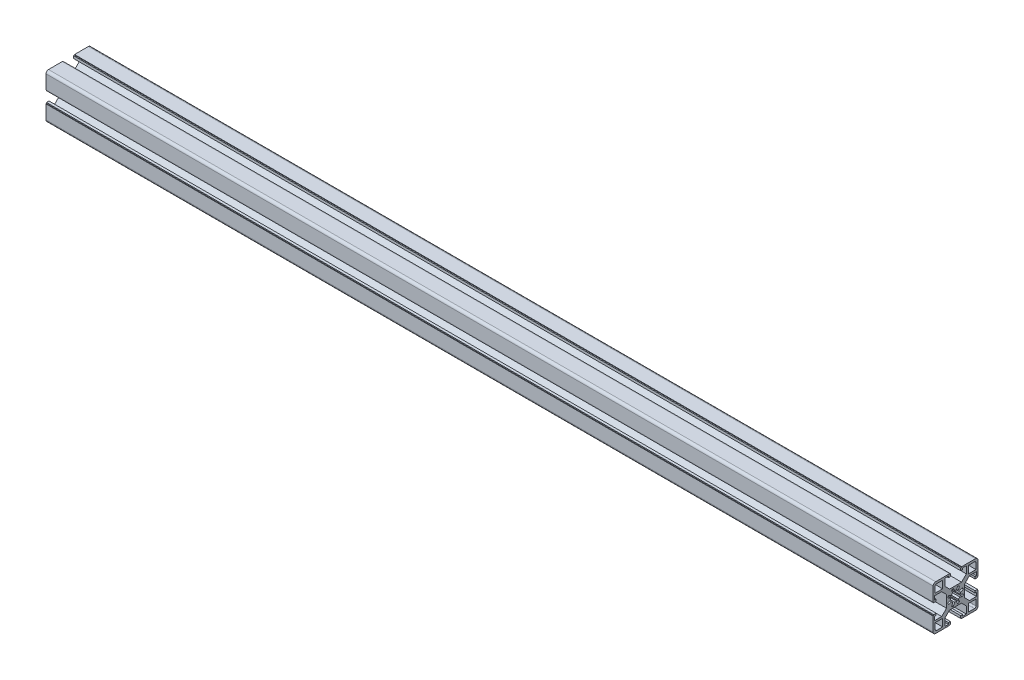
from build123d import *

# Parameters (mm, degrees)
ALUMINUM_PROFILE_45_X_45L_X_R2_5_1_DEPTH = 890


with BuildPart() as part:
    # Sketch1 → Aluminum Profile 45 X 45L X R2.5(1) (new body)
    with BuildSketch(Plane.YZ):
        with BuildLine():
            Line((6.1, -22.5), (20, -22.5))
            ThreePointArc((20, -22.5), (21.767766953, -21.767766953), (22.5, -20))
            Line((22.5, -20), (22.5, -6.1))
            Line((22.5, -6.1), (22, -6.1))
            Line((22, -6.1), (22, -5.1))
            Line((22, -5.1), (19.5, -5.1))
            Line((19.5, -5.1), (19.5, -7.1))
            Line((19.5, -7.1), (21, -7.1))
            Line((21, -7.1), (21, -10.8))
            Line((21, -10.8), (13.9, -10.8))
            Line((13.9, -10.8), (9.1, -6))
            Line((9.1, -6), (9.1, 6))
            Line((9.1, 6), (13.9, 10.8))
            Line((13.9, 10.8), (21, 10.8))
            Line((21, 10.8), (21, 7.1))
            Line((21, 7.1), (19.5, 7.1))
            Line((19.5, 7.1), (19.5, 5.1))
            Line((19.5, 5.1), (22, 5.1))
            Line((22, 5.1), (22, 6.1))
            Line((22, 6.1), (22.5, 6.1))
            Line((22.5, 6.1), (22.5, 20))
            ThreePointArc((22.5, 20), (21.767766953, 21.767766953), (20, 22.5))
            Line((20, 22.5), (6.1, 22.5))
            Line((6.1, 22.5), (6.1, 22))
            Line((6.1, 22), (5.1, 22))
            Line((5.1, 22), (5.1, 19.5))
            Line((5.1, 19.5), (7.1, 19.5))
            Line((7.1, 19.5), (7.1, 21))
            Line((7.1, 21), (10.8, 21))
            Line((10.8, 21), (10.8, 13.9))
            Line((10.8, 13.9), (6, 9.1))
            Line((6, 9.1), (-6, 9.1))
            Line((-6, 9.1), (-10.8, 13.9))
            Line((-10.8, 13.9), (-10.8, 21))
            Line((-10.8, 21), (-7.1, 21))
            Line((-7.1, 21), (-7.1, 19.5))
            Line((-7.1, 19.5), (-5.1, 19.5))
            Line((-5.1, 19.5), (-5.1, 22))
            Line((-5.1, 22), (-6.1, 22))
            Line((-6.1, 22), (-6.1, 22.5))
            Line((-6.1, 22.5), (-20, 22.5))
            ThreePointArc((-20, 22.5), (-21.767766953, 21.767766953), (-22.5, 20))
            Line((-22.5, 20), (-22.5, 6.1))
            Line((-22.5, 6.1), (-22, 6.1))
            Line((-22, 6.1), (-22, 5.1))
            Line((-22, 5.1), (-19.5, 5.1))
            Line((-19.5, 5.1), (-19.5, 7.1))
            Line((-19.5, 7.1), (-21, 7.1))
            Line((-21, 7.1), (-21, 10.8))
            Line((-21, 10.8), (-13.9, 10.8))
            Line((-13.9, 10.8), (-9.1, 6))
            Line((-9.1, 6), (-9.1, -6))
            Line((-9.1, -6), (-13.9, -10.8))
            Line((-13.9, -10.8), (-21, -10.8))
            Line((-21, -10.8), (-21, -7.1))
            Line((-21, -7.1), (-19.5, -7.1))
            Line((-19.5, -7.1), (-19.5, -5.1))
            Line((-19.5, -5.1), (-22, -5.1))
            Line((-22, -5.1), (-22, -6.1))
            Line((-22, -6.1), (-22.5, -6.1))
            Line((-22.5, -6.1), (-22.5, -20))
            ThreePointArc((-22.5, -20), (-21.767766953, -21.767766953), (-20, -22.5))
            Line((-20, -22.5), (-6.1, -22.5))
            Line((-6.1, -22.5), (-6.1, -22))
            Line((-6.1, -22), (-5.1, -22))
            Line((-5.1, -22), (-5.1, -19.5))
            Line((-5.1, -19.5), (-7.1, -19.5))
            Line((-7.1, -19.5), (-7.1, -21))
            Line((-7.1, -21), (-10.8, -21))
            Line((-10.8, -21), (-10.8, -13.9))
            Line((-10.8, -13.9), (-6, -9.1))
            Line((-6, -9.1), (6, -9.1))
            Line((6, -9.1), (10.8, -13.9))
            Line((10.8, -13.9), (10.8, -21))
            Line((10.8, -21), (7.1, -21))
            Line((7.1, -21), (7.1, -19.5))
            Line((7.1, -19.5), (5.1, -19.5))
            Line((5.1, -19.5), (5.1, -22))
            Line((5.1, -22), (6.1, -22))
            Line((6.1, -22), (6.1, -22.5))
        make_face()
        with BuildLine():
            Line((-12.8, 20.5), (-18.8, 20.5))
            ThreePointArc((-18.8, 20.5), (-19.860660172, 20.060660172), (-20.3, 19))
            Line((-20.3, 19), (-20.3, 13))
            Line((-20.3, 13), (-12.8, 13))
            Line((-12.8, 13), (-12.8, 20.5))
        make_face(mode=Mode.SUBTRACT)
        with BuildLine():
            Line((-20.3, -13), (-20.3, -19))
            ThreePointArc((-20.3, -19), (-19.860660172, -20.060660172), (-18.8, -20.5))
            Line((-18.8, -20.5), (-12.8, -20.5))
            Line((-12.8, -20.5), (-12.8, -13))
            Line((-12.8, -13), (-20.3, -13))
        make_face(mode=Mode.SUBTRACT)
        with BuildLine():
            Line((7.008352828, 3.985346991), (4.143383445, 2.798637817))
            ThreePointArc((4.143383445, 2.798637817), (3.535533906, 3.535533906), (2.798637817, 4.143383445))
            Line((2.798637817, 4.143383445), (3.985346991, 7.008352828))
            Line((3.985346991, 7.008352828), (2.137587926, 7.773719692))
            Line((2.137587926, 7.773719692), (0.950878752, 4.908750309))
            ThreePointArc((0.950878752, 4.908750309), (0, 5), (-0.950878752, 4.908750309))
            Line((-0.950878752, 4.908750309), (-2.137587926, 7.773719692))
            Line((-2.137587926, 7.773719692), (-3.985346991, 7.008352828))
            Line((-3.985346991, 7.008352828), (-2.798637817, 4.143383445))
            ThreePointArc((-2.798637817, 4.143383445), (-3.535533906, 3.535533906), (-4.143383445, 2.798637817))
            Line((-4.143383445, 2.798637817), (-7.008352828, 3.985346991))
            Line((-7.008352828, 3.985346991), (-7.773719692, 2.137587926))
            Line((-7.773719692, 2.137587926), (-4.908750309, 0.950878752))
            ThreePointArc((-4.908750309, 0.950878752), (-5, 0), (-4.908750309, -0.950878752))
            Line((-4.908750309, -0.950878752), (-7.773719692, -2.137587926))
            Line((-7.773719692, -2.137587926), (-7.008352828, -3.985346991))
            Line((-7.008352828, -3.985346991), (-4.143383445, -2.798637817))
            ThreePointArc((-4.143383445, -2.798637817), (-3.535533906, -3.535533906), (-2.798637817, -4.143383445))
            Line((-2.798637817, -4.143383445), (-3.985346991, -7.008352828))
            Line((-3.985346991, -7.008352828), (-2.137587926, -7.773719692))
            Line((-2.137587926, -7.773719692), (-0.950878752, -4.908750309))
            ThreePointArc((-0.950878752, -4.908750309), (0, -5), (0.950878752, -4.908750309))
            Line((0.950878752, -4.908750309), (2.137587926, -7.773719692))
            Line((2.137587926, -7.773719692), (3.985346991, -7.008352828))
            Line((3.985346991, -7.008352828), (2.798637817, -4.143383445))
            ThreePointArc((2.798637817, -4.143383445), (3.535533906, -3.535533906), (4.143383445, -2.798637817))
            Line((4.143383445, -2.798637817), (7.008352828, -3.985346991))
            Line((7.008352828, -3.985346991), (7.773719692, -2.137587926))
            Line((7.773719692, -2.137587926), (4.908750309, -0.950878752))
            ThreePointArc((4.908750309, -0.950878752), (5, 0), (4.908750309, 0.950878752))
            Line((4.908750309, 0.950878752), (7.773719692, 2.137587926))
            Line((7.773719692, 2.137587926), (7.008352828, 3.985346991))
        make_face(mode=Mode.SUBTRACT)
        with BuildLine():
            Line((20.3, -19), (20.3, -13))
            Line((20.3, -13), (12.8, -13))
            Line((12.8, -13), (12.8, -20.5))
            Line((12.8, -20.5), (18.8, -20.5))
            ThreePointArc((18.8, -20.5), (19.860660172, -20.060660172), (20.3, -19))
        make_face(mode=Mode.SUBTRACT)
        with BuildLine():
            Line((20.3, 13), (20.3, 19))
            ThreePointArc((20.3, 19), (19.860660172, 20.060660172), (18.8, 20.5))
            Line((18.8, 20.5), (12.8, 20.5))
            Line((12.8, 20.5), (12.8, 13))
            Line((12.8, 13), (20.3, 13))
        make_face(mode=Mode.SUBTRACT)
    extrude(amount=ALUMINUM_PROFILE_45_X_45L_X_R2_5_1_DEPTH)


solid = part.part
